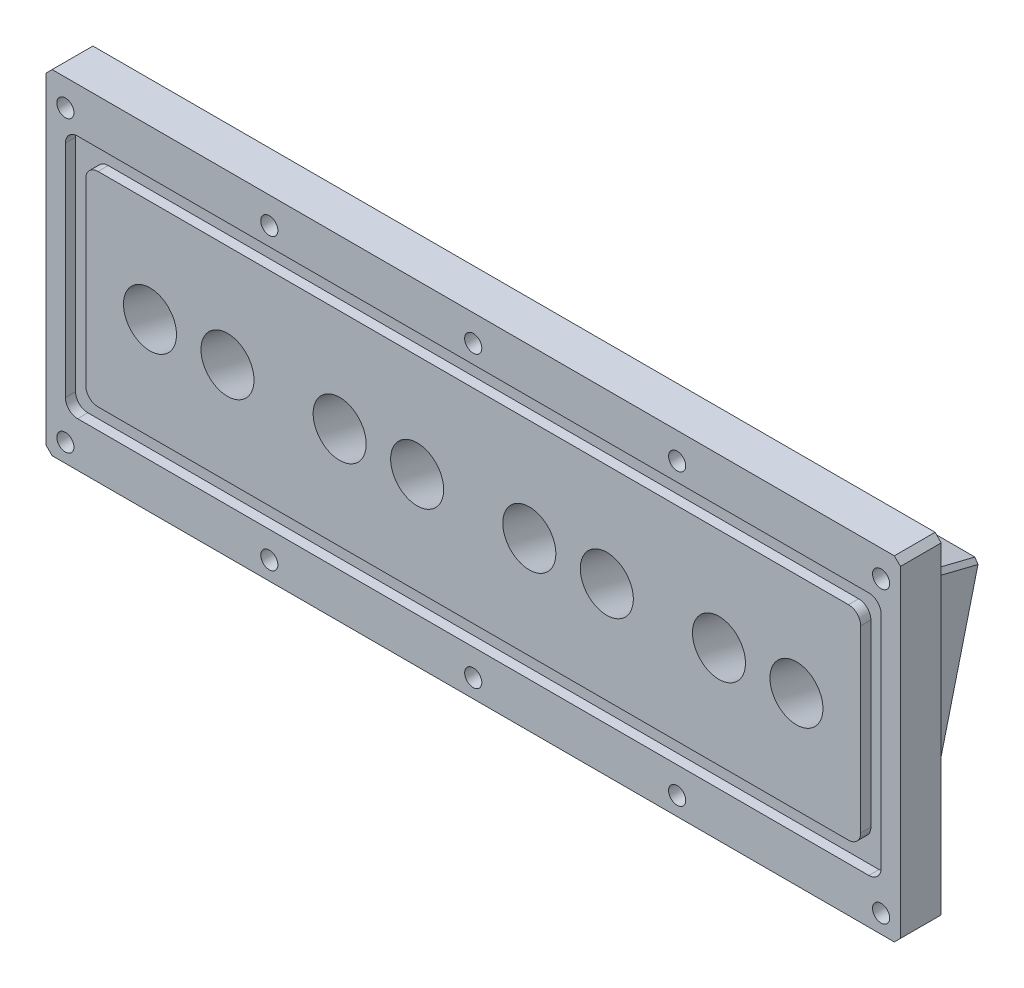
from build123d import *

# Parameters (mm, degrees)
SKETCH1_W             = 419
SKETCH1_H             = 164
BOSS_EXTRUDE1_DEPTH   = 20
SKETCH2_W             = 400
SKETCH2_H             = 120
SKETCH2_W_2           = 380
SKETCH2_H_2           = 100
CUT_EXTRUDE1_DEPTH    = 5
FILLET1_R             = 6
CHAMFER1_SIZE         = 3
HOLE1_D               = 8.4
HOLE1_CBORE_D         = 15
HOLE1_CBORE_DEPTH     = 11
BOSS_EXTRUDE2_DEPTH   = 379
CHAMFER2_SIZE         = 2
HOLE2_D               = 26
M6_TAPPED_HOLE1_D     = 5
M6_TAPPED_HOLE1_DEPTH = 12
M6_TAPPED_HOLE1_TIP   = 1.502151548
SKETCH12_W            = 359
SKETCH12_H            = 78
CUT_EXTRUDE2_DEPTH    = 15
FILLET2_R             = 6


with BuildPart() as part:
    # Sketch1 → Boss-Extrude1 (new body)
    with BuildSketch(Plane.XY):
        Rectangle(SKETCH1_W, SKETCH1_H)
    extrude(amount=BOSS_EXTRUDE1_DEPTH)

    # Sketch2 → Cut-Extrude1 (cut)
    with BuildSketch(Plane.XY.offset(20)):
        Rectangle(SKETCH2_W, SKETCH2_H)
        Rectangle(SKETCH2_W_2, SKETCH2_H_2, mode=Mode.SUBTRACT)
    extrude(amount=-CUT_EXTRUDE1_DEPTH, mode=Mode.SUBTRACT)

    # Fillet1
    fillet1_edges = [part.edges().sort_by_distance(p)[0] for p in [
        (200, 60, 17.5),
        (200, -60, 17.5),
        (-200, -60, 17.5),
        (-200, 60, 17.5),
        (190, -50, 17.5),
        (-190, -50, 17.5),
        (-190, 50, 17.5),
        (190, 50, 17.5),
    ]]
    fillet(fillet1_edges, radius=FILLET1_R)

    # Chamfer1
    chamfer1_edges = [part.edges().sort_by_distance(p)[0] for p in [
        (209.5, -82, 10),
        (-209.5, -82, 10),
        (-209.5, 82, 10),
        (209.5, 82, 10),
    ]]
    chamfer(chamfer1_edges, length=CHAMFER1_SIZE)

    # Hole1 (through all)
    with Locations(Plane(origin=(0, 0, 0), x_dir=(-1, 0, 0), z_dir=(0, 0, -1))):
        with Locations((-200, 69), (-200, -73), (-100, -73), (0, -73), (100, -73), (200, -73), (200, 69), (100, 69), (0, 69), (-100, 69)):
            CounterBoreHole(HOLE1_D / 2, HOLE1_CBORE_D / 2, HOLE1_CBORE_DEPTH)

    # Sketch6 → Boss-Extrude2 (add)
    with BuildSketch(Plane.ZY.offset(189.5)):
        Polygon((0, 52.33), (-38.51, 42.73252989), (-11.898591484, -64), (0, -64), align=None)
    extrude(amount=-BOSS_EXTRUDE2_DEPTH)

    # Chamfer2
    chamfer2_edges = [part.edges().sort_by_distance(p)[0] for p in [
        (189.5, -64, -5.949295742),
        (189.5, 47.531264945, -19.255),
        (-189.5, 47.531264945, -19.255),
        (-189.5, -64, -5.949295742),
    ]]
    chamfer(chamfer2_edges, length=CHAMFER2_SIZE)

    # Hole2 (through all)
    with Locations(Plane(origin=(0, -6.538702198, -26.225302106), x_dir=(-1, 0, 0), z_dir=(0, -0.24192189559966124, -0.970295726275998))):
        with Locations((158.5, -4.924424644), (120.501104945, -5.214208356), (65.5, -4.924424644), (27.501104945, -5.214208356), (-27.5, -4.924424644), (-65.498895055, -5.214208356), (-120.5, -4.924424644), (-158.498895055, -5.214208356)):
            Hole(HOLE2_D / 2)

    # M6 Tapped Hole1
    with Locations(Plane(origin=(0, -6.538702198, -26.225302106), x_dir=(-1, 0, 0), z_dir=(0, -0.24192189559966124, -0.970295726275998))):
        with Locations((-169.5, 40.075575356), (-109.5, 40.075575356), (-76.5, 40.075575356), (-16.5, 40.075575356), (16.5, 40.075575356), (76.5, 40.075575356), (109.5, 40.075575356), (169.5, 40.075575356), (169.5, -49.924424644), (109.5, -49.924424644), (76.5, -49.924424644), (16.5, -49.924424644), (-16.5, -49.924424644), (-76.5, -49.924424644), (-109.5, -49.924424644), (-169.5, -49.924424644)):
            Hole(M6_TAPPED_HOLE1_D / 2, depth=M6_TAPPED_HOLE1_DEPTH)
            with Locations((0, 0, -(M6_TAPPED_HOLE1_DEPTH + M6_TAPPED_HOLE1_TIP / 2))):  # 118° drill point
                Cone(0, M6_TAPPED_HOLE1_D / 2, M6_TAPPED_HOLE1_TIP, mode=Mode.SUBTRACT)

    # Sketch12 → Cut-Extrude2 (cut)
    with BuildSketch(Plane(origin=(0, -6.538702198, -26.225302106), x_dir=(-1, 0, 0), z_dir=(0, -0.24192189559966124, -0.970295726275998))):
        with Locations((0, -4.920396675)):
            Rectangle(SKETCH12_W, SKETCH12_H)
    extrude(amount=-CUT_EXTRUDE2_DEPTH, mode=Mode.SUBTRACT)

    # Fillet2
    fillet2_edges = [part.edges().sort_by_distance(p)[0] for p in [
        (179.5, -47.340061171, -8.32277854),
        (179.5, 28.343005479, -27.192686396),
        (-179.5, 28.343005479, -27.192686396),
        (-179.5, -47.340061171, -8.32277854),
    ]]
    fillet(fillet2_edges, radius=FILLET2_R)


solid = part.part
